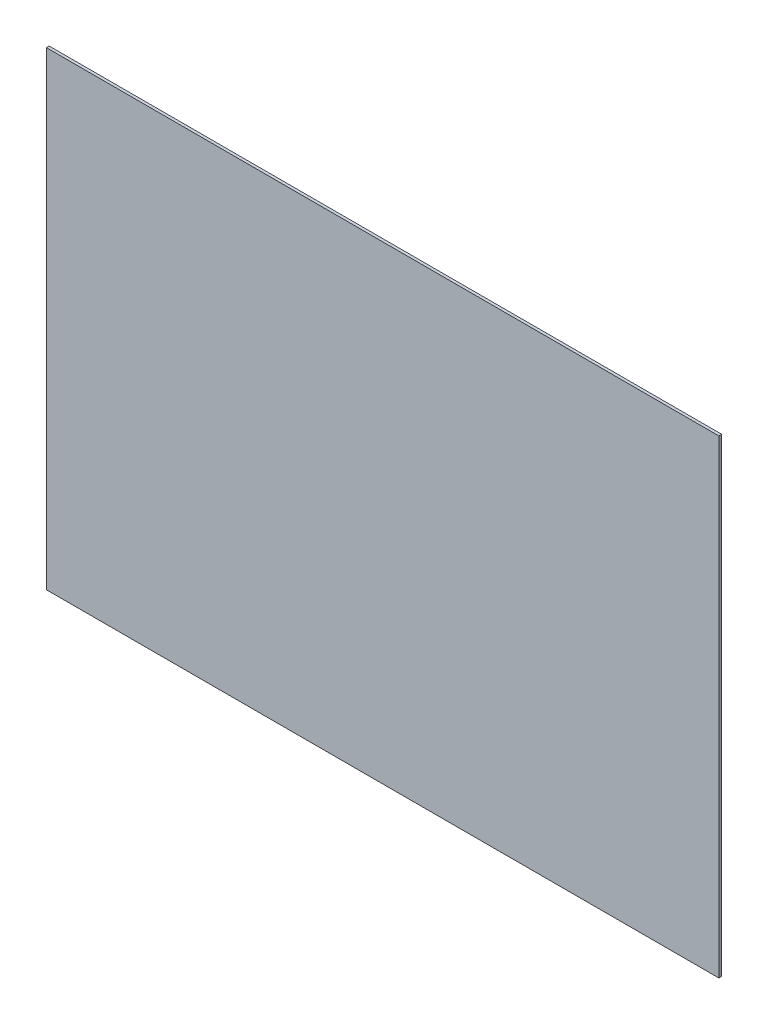
from build123d import *

# Parameters (mm, degrees)
SKETCH_1_W      = 1206
SKETCH_1_H      = 842
EXTRUDE_1_DEPTH = 5


with BuildPart() as part:
    # 草图1 → 凸台-拉伸1 (new body)
    with BuildSketch(Plane.XY):
        Rectangle(SKETCH_1_W, SKETCH_1_H)
    extrude(amount=EXTRUDE_1_DEPTH)


solid = part.part
